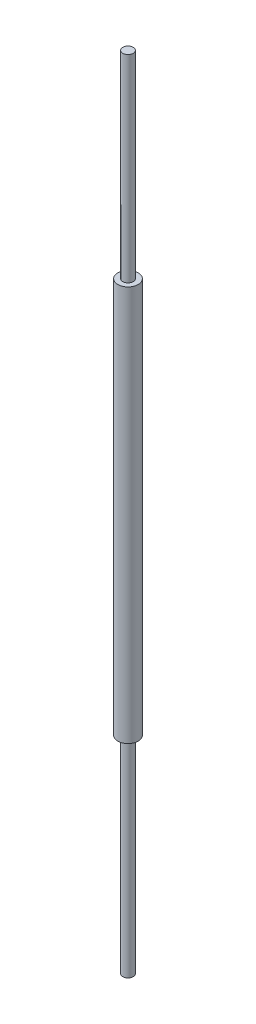
from build123d import *


with BuildPart() as part:
    # Sketch1 → Revolve1 (revolve)
    with BuildSketch(Plane(origin=(0, 0, 0), x_dir=(0, 0, -1), z_dir=(1, 0, 0))):
        Polygon((0.45, 16), (0.875, 16), (0.875, 50), (0.45, 50), (0.45, 67), (0, 67), (0, -1.75), (0.45, -1.75), align=None)
    revolve(axis=Axis((0, -4.379065135, 0), (0, 1, 0)))


solid = part.part
